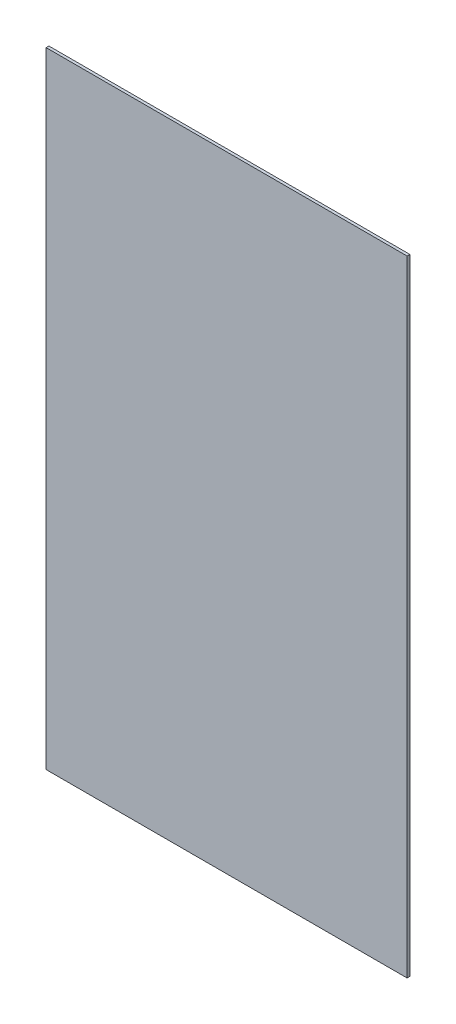
from build123d import *

# Parameters (mm, degrees)
SKETCH_1_W      = 646
SKETCH_1_H      = 1119
EXTRUDE_1_DEPTH = 5


with BuildPart() as part:
    # 草图1 → 凸台-拉伸1 (new body)
    with BuildSketch(Plane.XY):
        Rectangle(SKETCH_1_W, SKETCH_1_H)
    extrude(amount=EXTRUDE_1_DEPTH)


solid = part.part
